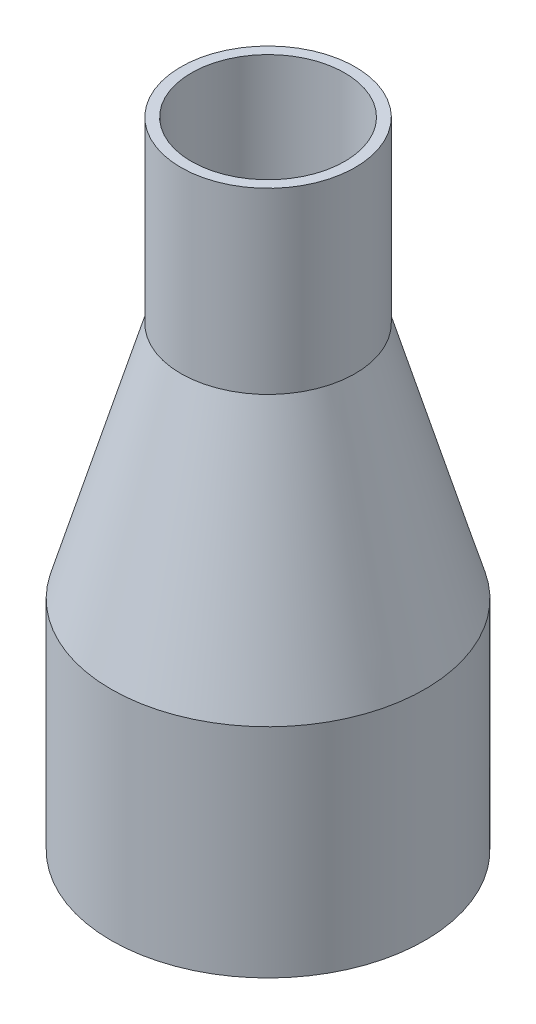
SolidWorks part; units mm, degrees
ref_plane "Front Plane" through (0, 0, 0) normal (0, 0, 1) x (1, 0, 0)
ref_plane "Top Plane" through (0, 0, 0) normal (0, 1, 0) x (1, 0, 0)
ref_plane "Right Plane" through (0, 0, 0) normal (1, 0, 0) x (0, 0, -1)
sketch "Sketch 1" plane through (0, 0, 0) normal (0, 0, 1) x (1, 0, 0)
  line L0 (0, 22.2458) -> (0, -27.7542) construction
  line L1 (-29.2373, 0) -> (22.0339, 0) construction
  line L2 (-12.5, 45.5) -> (-12.5, 19.9)
  line L3 (-12.5, 19.9) -> (-22.5, -14.3)
  line L4 (-22.5, -14.3) -> (-22.5, -45.5)
  line L5 (-11, 45.5) -> (-11, 19.6852)
  line L6 (-11, 19.6852) -> (-21, -14.5148)
  line L7 (-21, -14.5148) -> (-21, -45.5)
  line L8 (-22.5, -45.5) -> (-21, -45.5)
  line L9 (-12.5, 45.5) -> (-11, 45.5)
  dimension "D1" = 25
  dimension "D2" = 45
  dimension "D3" = 31.2
  dimension "D4" = 91
  dimension "D6" = 25.6
  dimension "D5" = 1.5
revolve "Revolve 1" add sketch "Sketch 1" angle 360 about L0
